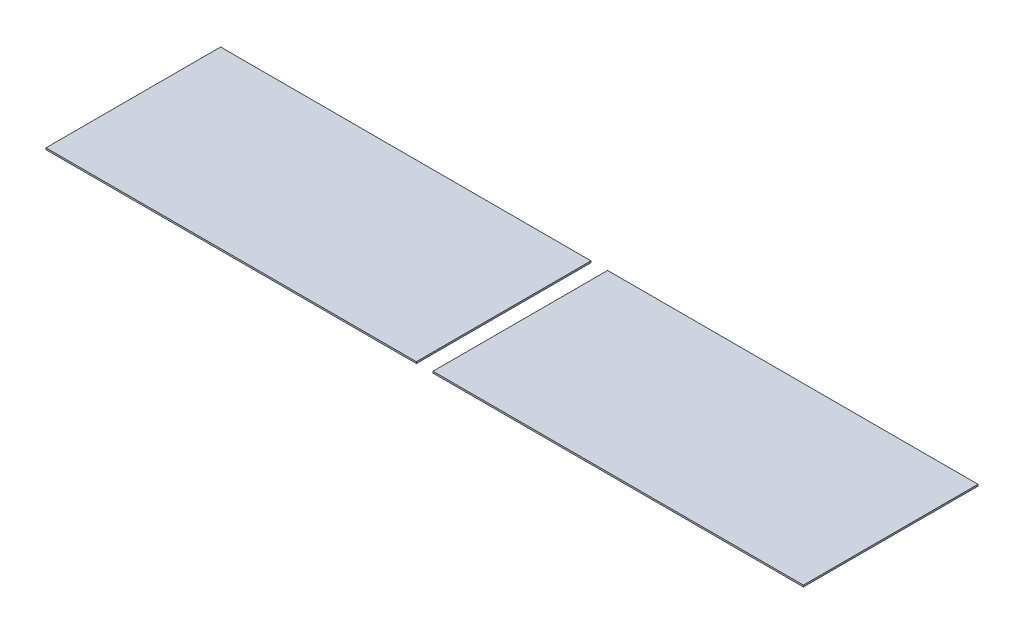
SolidWorks part; units mm, degrees
material "Q235"
ref_plane "Front Plane" through (0, 0, 0) normal (0, 0, 1) x (1, 0, 0)
ref_plane "Top Plane" through (0, 0, 0) normal (0, 1, 0) x (1, 0, 0)
ref_plane "Right Plane" through (0, 0, 0) normal (1, 0, 0) x (0, 0, -1)
sketch "Sketch1" plane through (0, 0, 0) normal (0, 1, 0) x (1, 0, 0)
  line L1 (-911, 210) -> (911, 210)
  line L2 (-911, 210) -> (-911, -210)
  line L3 (-911, -210) -> (911, -210)
  line L4 (911, 210) -> (911, -210)
  line L5 (-911, 210) -> (911, -210) construction
  line L6 (-911, -210) -> (911, 210) construction
  point P0 (0, 0)
  dimension "D1" = 420
  dimension "D2" = 1822
extrude "Boss-Extrude1" add sketch "Sketch1" along normal blind 4
sketch "Sketch2" plane through (0, 4, 0) normal (0, 1, 0) x (1, 0, 0)
  line L0 (911, 210) -> (-911, 210) construction
  line L1 (-871, 210) -> (-751, 210)
  line L2 (-871, 210) -> (-871, 160)
  line L3 (-871, 160) -> (-751, 160)
  line L4 (-751, 210) -> (-751, 160)
  line L5 (0, 0) -> (0, 210) construction
  line L6 (751, 210) -> (751, 160)
  line L7 (871, 160) -> (751, 160)
  line L8 (871, 210) -> (871, 160)
  line L9 (871, 210) -> (751, 210)
  line L10 (-911, 210) -> (-911, -210) construction
  dimension "D1" = 50
  dimension "D2" = 120
  dimension "D3" = 40
extrude "Cut-Extrude1" [suppressed] cut sketch "Sketch2" against normal blind 4
sketch "Sketch3" plane through (0, 4, 0) normal (0, 1, 0) x (1, 0, 0)
  line L0 (911, 210) -> (-911, 210) construction
  line L1 (-300, 210) -> (-180, 210)
  line L2 (-300, 210) -> (-300, 160)
  line L3 (-300, 160) -> (-180, 160)
  line L4 (-180, 210) -> (-180, 160)
  line L5 (0, 0) -> (0, 176.2033) construction
  line L6 (180, 210) -> (180, 160)
  line L7 (300, 160) -> (180, 160)
  line L8 (300, 210) -> (300, 160)
  line L9 (300, 210) -> (180, 210)
  dimension "D1" = 360
  dimension "D2" = 120
  dimension "D3" = 50
extrude "Cut-Extrude2" [suppressed] cut sketch "Sketch3" against normal blind 4
sketch "Sketch5" [suppressed] plane through (0, 4, 0) normal (0, 1, 0) x (1, 0, 0)
  line L0 (-300, 225) -> (-755, 225) construction
  line L1 (-725, 225) -> (-545, 225)
  line L2 (-725, 225) -> (-725, 195)
  line L3 (-725, 195) -> (-545, 195)
  line L4 (-545, 225) -> (-545, 195)
  line L5 (0, 0) -> (0, 225) construction
  line L6 (180, 225) -> (-180, 225) construction
  line L7 (545, 225) -> (545, 195)
  line L8 (725, 195) -> (545, 195)
  line L9 (725, 225) -> (725, 195)
  line L10 (725, 225) -> (545, 225)
  line L11 (-755, 175) -> (-755, 225) construction
  dimension "D1" = 30
  dimension "D2" = 180
  dimension "D3" = 30
extrude "Cut-Extrude3" [suppressed] cut sketch "Sketch5" against normal blind 4
sketch "Sketch6" [suppressed] plane through (0, 4, 0) normal (0, 1, 0) x (1, 0, 0)
  line L1 (-725, 195) -> (-793.4337, 195)
  line L2 (-725, 195) -> (-725, 272.6372)
  line L3 (-725, 272.6372) -> (-793.4337, 272.6372)
  line L4 (-793.4337, 195) -> (-793.4337, 272.6372)
  line L5 (725, 195) -> (786.5821, 195)
  line L6 (725, 195) -> (725, 264.6233)
  line L7 (725, 264.6233) -> (786.5821, 264.6233)
  line L8 (786.5821, 195) -> (786.5821, 264.6233)
extrude "Cut-Extrude4" [suppressed] cut sketch "Sketch6" against normal through all
sketch "Sketch7" plane through (0, 4, 0) normal (0, 1, 0) x (1, 0, 0)
  line L1 (-20, 286.8884) -> (20, 286.8884)
  line L2 (-20, 286.8884) -> (-20, -286.8884)
  line L3 (-20, -286.8884) -> (20, -286.8884)
  line L4 (20, 286.8884) -> (20, -286.8884)
  line L5 (-20, 286.8884) -> (20, -286.8884) construction
  line L6 (-20, -286.8884) -> (20, 286.8884) construction
  point P0 (0, 0)
  dimension "D1" = 40
extrude "Cut-Extrude5" cut sketch "Sketch7" against normal through all
